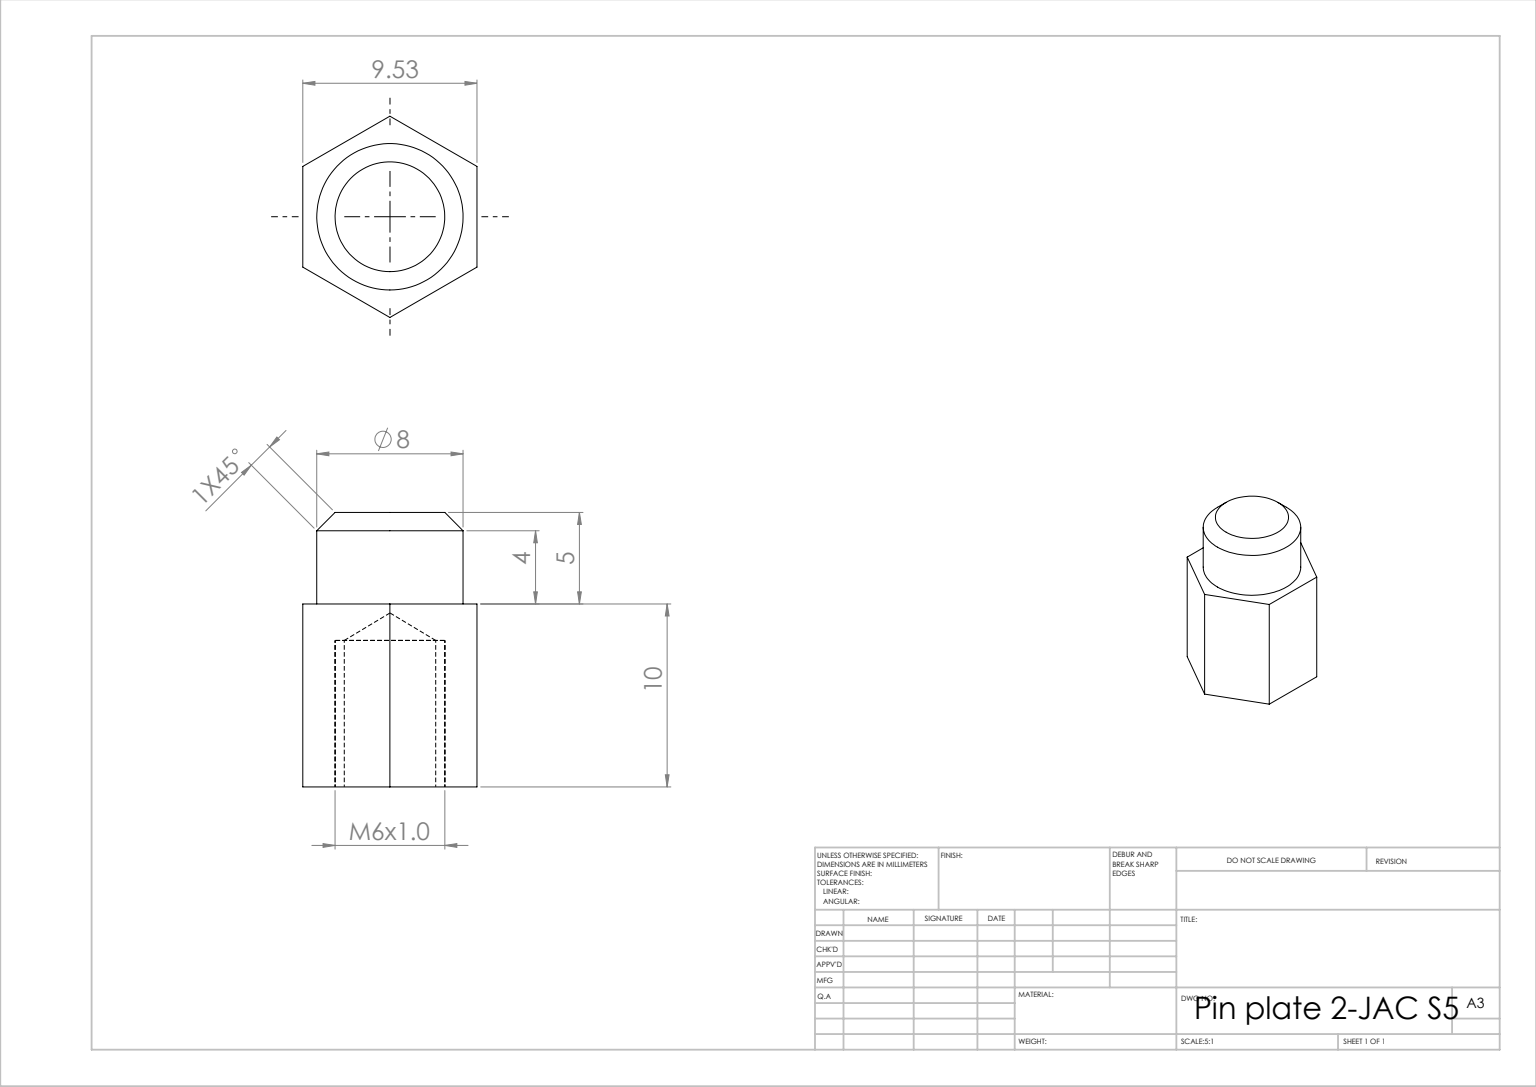
from build123d import *

# Parameters (mm, degrees)
BOSS_EXTRUDE1_DEPTH            = 5
SKETCH3_R                      = 4
BOSS_EXTRUDE2_DEPTH            = 5
CHAMFER1_SIZE                  = 1
M6X1_0_TAPPED_HOLE2_AT_2_COUNT = 2
M6X1_0_TAPPED_HOLE2_AT_2_PITCH = 0.000121298


with BuildPart() as part:
    # Sketch1 → Boss-Extrude1 (new, symmetric)
    with BuildSketch(Plane(origin=(0, 0, 0), x_dir=(1, 0, 0), z_dir=(0, 1, 0))):
        Polygon((0, 5.5), (-4.763139721, 2.75), (-4.763139721, -2.75), (0, -5.5), (4.763139721, -2.75), (4.763139721, 2.75), align=None)
    extrude(amount=BOSS_EXTRUDE1_DEPTH, both=True)

    # Sketch3 → Boss-Extrude2 (add)
    with BuildSketch(Plane(origin=(0, 5, 0), x_dir=(1, 0, 0), z_dir=(0, 1, 0))):
        with Locations(Location((0, 0, 0), (0, 0, 270))):
            Circle(SKETCH3_R)
    extrude(amount=BOSS_EXTRUDE2_DEPTH)

    # Chamfer1
    chamfer1_edges = [part.edges().sort_by_distance(p)[0] for p in [
        (0, 10, -4),
    ]]
    chamfer(chamfer1_edges, length=CHAMFER1_SIZE)

    # Sketch19 → M6x1.0 Tapped Hole2 (revolve, cut)
    with BuildSketch(Plane(origin=(-7.813e-06, -5, 0.000121047), x_dir=(0, 0, -1), z_dir=(1, 0, 0))):
        Polygon((0, 0), (0, 9.502151548), (2.5, 8), (2.5, 0), align=None)
    m6x1_0_tapped_hole2 = revolve(axis=Axis((-7.813e-06, -11.35, 0.000121047), (0, 1, 0)), mode=Mode.SUBTRACT)

    # M6x1.0 Tapped Hole2 at 2: M6x1.0 Tapped Hole2 ×2
    with Locations(*[Vector(0.06441225047789163, 0, -0.9979233748080929) * (i * M6X1_0_TAPPED_HOLE2_AT_2_PITCH) for i in range(1, M6X1_0_TAPPED_HOLE2_AT_2_COUNT)]):
        add(m6x1_0_tapped_hole2, mode=Mode.SUBTRACT)


solid = part.part
